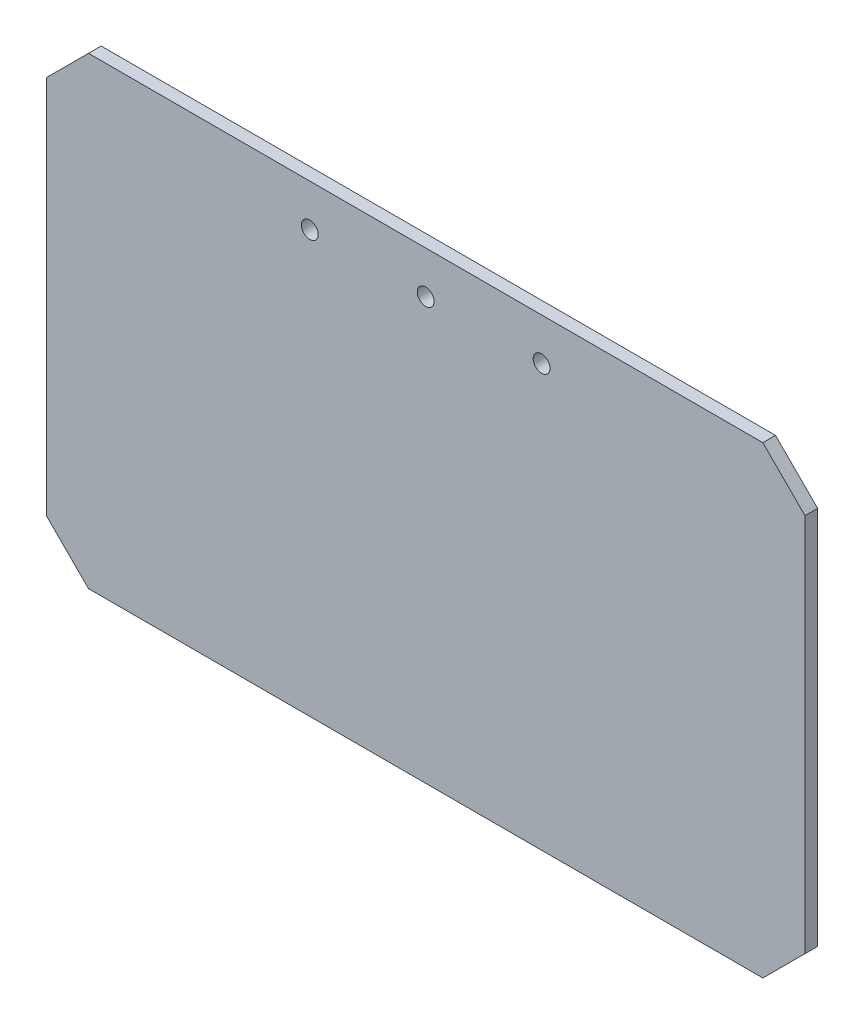
SolidWorks part; units mm, degrees
material "普通碳钢"
ref_plane "Front Plane" through (0, 0, 0) normal (0, 0, 1) x (1, 0, 0)
ref_plane "Top Plane" through (0, 0, 0) normal (0, 1, 0) x (1, 0, 0)
ref_plane "Right Plane" through (0, 0, 0) normal (1, 0, 0) x (0, 0, -1)
sketch "Sketch1" plane through (0, 0, 0) normal (0, 0, 1) x (1, 0, 0)
  line L0 (90, -5) -> (90, -81.335) construction
  line L1 (10, 0) -> (170, 0)
  line L2 (0, -10) -> (0, -100)
  line L3 (10, -110) -> (170, -110)
  line L4 (180, -10) -> (180, -100)
  line L5 (0, 0) -> (180, -110) construction
  line L6 (0, -110) -> (180, 0) construction
  line L7 (10, 0) -> (0, -10)
  line L8 (170, 0) -> (180, -10)
  line L9 (180, -100) -> (170, -110)
  line L10 (0, -100) -> (10, -110)
  circle A0 centre (90, -10) radius 2
  circle A1 centre (117.5, -10) radius 2
  circle A2 centre (62.5, -10) radius 2
  point P4 (90, -55)
  dimension "D3" = 4
  dimension "D1" = 180
  dimension "D2" = 110
  dimension "D4" = 27.5
  dimension "D5" = 27.5
  dimension "D6" = 10
extrude "Boss-Extrude1" add sketch "Sketch1" along normal blind 3
cosmetic thread "Cosmetic Thread1" parameters "D2"=5
cosmetic thread "Cosmetic Thread2" parameters "D2"=5
cosmetic thread "Cosmetic Thread3" parameters "D2"=5
